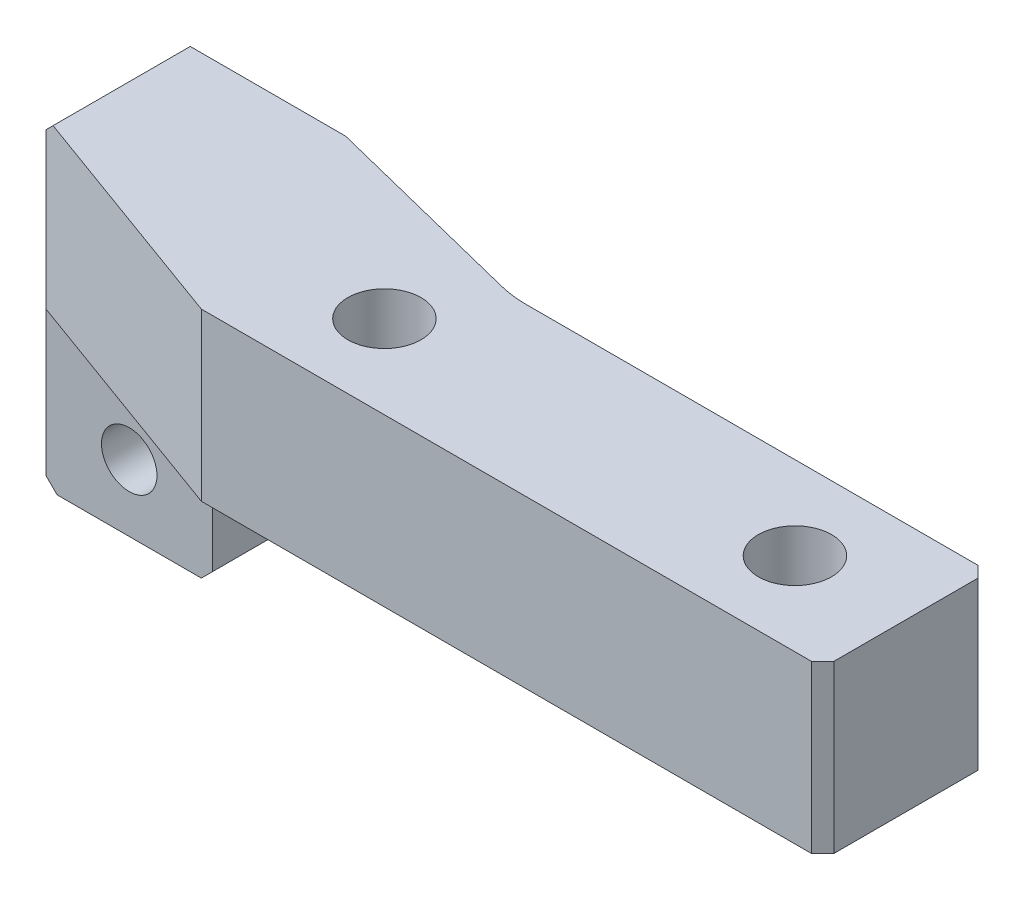
from build123d import *

# Parameters (mm, degrees)
SKETCH_1_W                   = 78
SKETCH_1_H                   = 15
EXTRUDE_1_DEPTH              = 7.5
HOLE_WIZARD_M6_1_D           = 6.6
HOLE_WIZARD_M6_1_CBORE_D     = 11
HOLE_WIZARD_M6_1_CBORE_DEPTH = 6.8
EXTRUDE_3_DEPTH              = 15
SKETCH_2_W                   = 15
SKETCH_2_H                   = 12
EXTRUDE_2_DEPTH              = 14
HOLE_WIZARD_M6_1_2_D         = 5
CUT_EXTRUDE_1_DEPTH          = 51.182168148
CHAMFER_1_SIZE               = 1
FILLET_2_R                   = 10


with BuildPart() as part:
    # 草图1 → 凸台-拉伸1 (new, symmetric)
    with BuildSketch(Plane(origin=(0, 0, 0), x_dir=(1, 0, 0), z_dir=(0, 1, 0))):
        Rectangle(SKETCH_1_W, SKETCH_1_H)
    extrude(amount=EXTRUDE_1_DEPTH, both=True)

    # Hole Wizard M6 _1 (through all)
    with Locations(Plane.XZ.offset(7.5)):
        with Locations((29, 0), (-8, 0)):
            CounterBoreHole(HOLE_WIZARD_M6_1_D / 2, HOLE_WIZARD_M6_1_CBORE_D / 2, HOLE_WIZARD_M6_1_CBORE_DEPTH)

    # 草图8 → 凸台-拉伸3 (add)
    with BuildSketch(Plane(origin=(0, 7.5, 0), x_dir=(1, 0, 0), z_dir=(0, 1, 0))):
        Polygon((-24, 12.5), (-39, 12.5), (-39, 7.5), (-4, 7.5), align=None)
    extrude(amount=-EXTRUDE_3_DEPTH)

    # 草图2 → 凸台-拉伸2 (add)
    with BuildSketch(Plane(origin=(0, -7.5, 0), x_dir=(1, 0, 0), z_dir=(0, 1, 0))):
        with Locations((-31.5, 6.5)):
            Rectangle(SKETCH_2_W, SKETCH_2_H)
    extrude(amount=-EXTRUDE_2_DEPTH)

    # Hole Wizard M6 _1 2 (through all)
    with Locations(Plane(origin=(-28.5, 0, -0.5), x_dir=(1, 0, 0), z_dir=(0, 0, 1))):
        with Locations((-3, -15.5)):
            Hole(HOLE_WIZARD_M6_1_2_D / 2)

    # 草图9 → 切除-拉伸1 (cut, through all)
    with BuildSketch(Plane(origin=(0, -21.5, 0), x_dir=(-1, 0, 0), z_dir=(0, -1, 0))):
        Polygon((39, 0.5), (39, -7.5), (17, -7.5), align=None)
    extrude(amount=-CUT_EXTRUDE_1_DEPTH, mode=Mode.SUBTRACT)

    # 倒角1
    chamfer_1_edges = [part.edges().sort_by_distance(p)[0] for p in [
        (-39, 7.5, -6.5),
        (-39, -21.5, -6.5),
        (-24, -21.5, -6.5),
        (39, 0, 7.5),
        (39, 0, -7.5),
    ]]
    chamfer(chamfer_1_edges, length=CHAMFER_1_SIZE)

    # 圆角2
    fillet_2_edges = [part.edges().sort_by_distance(p)[0] for p in [
        (-4, 0, -7.5),
    ]]
    fillet(fillet_2_edges, radius=FILLET_2_R)


solid = part.part
